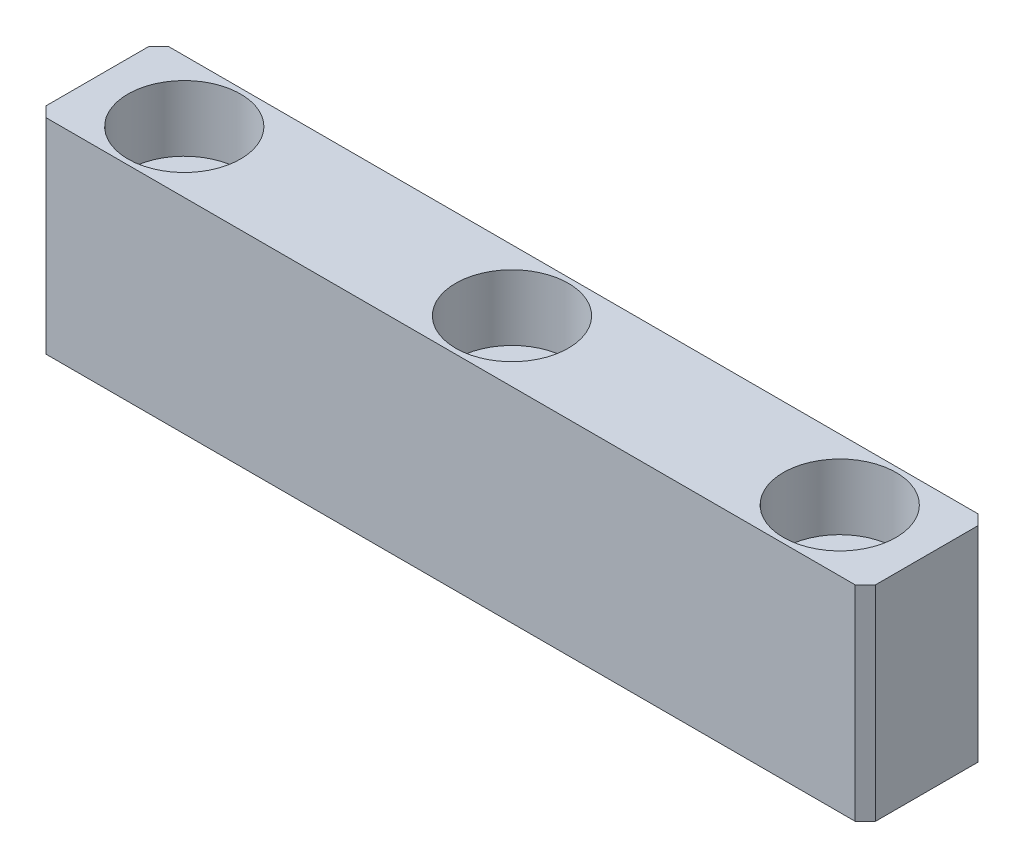
SolidWorks part; units mm, degrees
material "6061Al"
ref_plane "前视基准面" through (0, 0, 0) normal (0, 0, 1) x (1, 0, 0)
ref_plane "上视基准面" through (0, 0, 0) normal (0, 1, 0) x (1, 0, 0)
ref_plane "右视基准面" through (0, 0, 0) normal (1, 0, 0) x (0, 0, -1)
sketch "草图1" plane through (0, 0, 0) normal (0, 0, 1) x (1, 0, 0)
  line L1 (-40.5, -10) -> (40.5, -10)
  line L2 (-40.5, -10) -> (-40.5, 10)
  line L3 (-40.5, 10) -> (40.5, 10)
  line L4 (40.5, -10) -> (40.5, 10)
  line L5 (-40.5, -10) -> (40.5, 10) construction
  line L6 (-40.5, 10) -> (40.5, -10) construction
  point P0 (0, 0)
  dimension "D1" = 81
  dimension "D2" = 20
extrude "凸台-拉伸1" add sketch "草图1" along normal blind 12
hole_wizard "M6 六角凹头螺钉的柱形沉头孔1" positions "草图2" profile "草图3" counterbore size "M6" standard "ISO" end condition through all
sketch "草图2" plane through (0, 10, 0) normal (0, 1, 0) x (1, 0, 0)
  line L0 (0, 0) -> (0, -12) construction
  line L1 (40.5, -12) -> (-40.5, -12) construction
  line L3 (-40.5, -12) -> (-40.5, 0) construction
  point P0 (-32, -6)
  point P2 (0, -6)
  point P4 (32, -6)
  dimension "D1" = 8.5
sketch "草图3" plane through (-32, 10, 6) normal (1, 0, 0) x (0, 0, 1)
  line L0 (0, 0) -> (0, 20)
  line L1 (0, 20) -> (3.3, 20)
  line L3 (3.3, 20) -> (3.3, 6.4)
  line L4 (3.3, 6.4) -> (5.5, 6.4)
  line L5 (5.5, 6.4) -> (5.5, 0)
  line L7 (5.5, 0) -> (0, 0)
  line L11 (0, -6.35) -> (0, 107.95) construction
  dimension "通孔孔直径" = 6.6
  dimension "通孔孔深度" = 20
  dimension "柱形沉头孔直径" = 11
  dimension "柱形沉头孔深度" = 6.4
chamfer "倒角1" distance 1 angle 45 4 edges at (40.5, 0, 12) (40.5, 0, 0) (-40.5, 0, 0) (-40.5, 0, 12)
